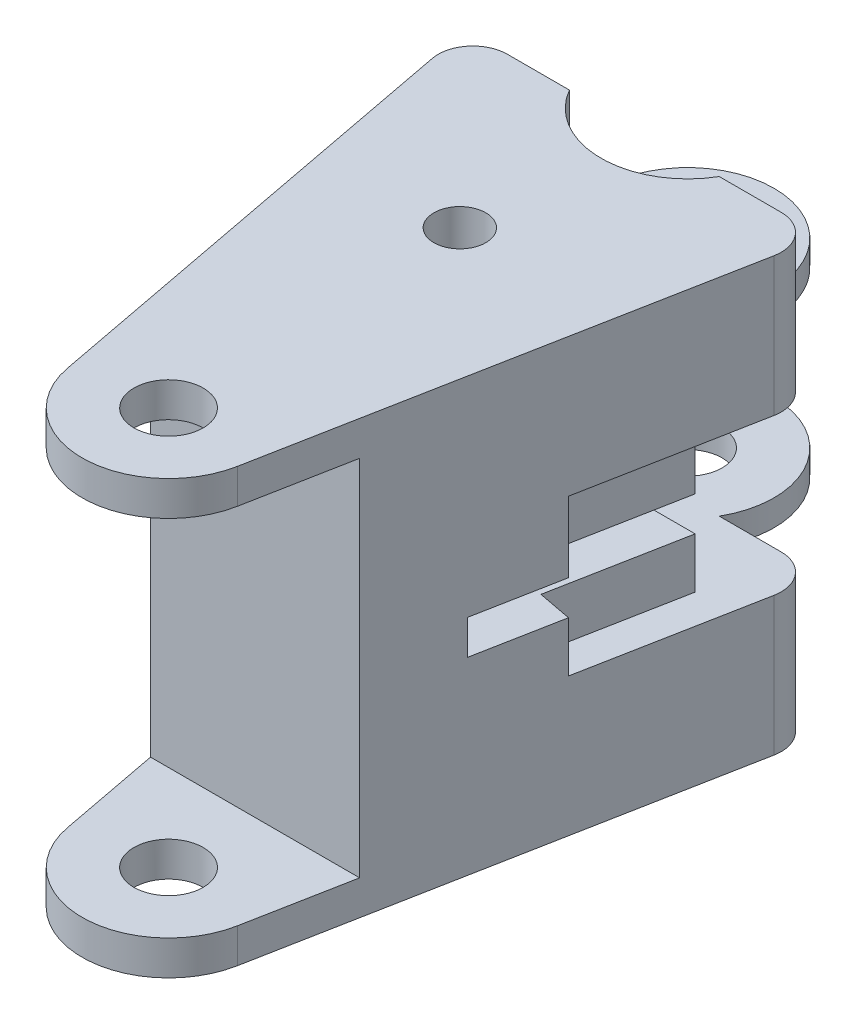
SolidWorks part; units mm, degrees
ref_plane "Front Plane" through (0, 0, 0) normal (0, 0, 1) x (1, 0, 0)
ref_plane "Top Plane" through (0, 0, 0) normal (0, 1, 0) x (1, 0, 0)
ref_plane "Right Plane" through (0, 0, 0) normal (1, 0, 0) x (0, 0, -1)
other "Configuration Table"
sketch "Sketch1" plane through (0, 0, 0) normal (0, 1, 0) x (1, 0, 0)
  line L0 (-4.3301, -2.5) -> (-10.3301, -2.5)
  line L1 (-10.3301, -2.5) -> (-4.9116, -30.9359)
  line L2 (0, 0) -> (0, -50000) construction
  line L3 (10.3301, -2.5) -> (4.9116, -30.9359)
  line L4 (4.3301, -2.5) -> (10.3301, -2.5)
  arc A0 (4.3301, -2.5) -> (-4.3301, -2.5) centre (0, 0) ccw
  arc A1 (-4.9116, -30.9359) -> (4.9116, -30.9359) centre (0, -30) ccw
  dimension "D1" = 10
  dimension "D2" = 10
  dimension "D3" = 30
  dimension "D4" = 6
  dimension "D5" = 2.5
extrude "Boss-Extrude1" add sketch "Sketch1" along normal blind 25
sketch "Sketch2" plane through (0, 25, 0) normal (0, 1, 0) x (1, 0, 0)
  circle A0 centre (0, 0) radius 2
  circle A1 centre (0, -30) radius 2
  dimension "D1" = 4
  dimension "D2" = 4
extrude "Cut-Extrude1" cut sketch "Sketch2" against normal through all
fillet "Fillet1" radius 2 1 edges at (10.3301, 12.5, 2.5)
fillet "Fillet2" radius 2 1 edges at (-10.3301, 12.5, 2.5)
sketch "Sketch3" plane through (0, 25, 0) normal (0, 1, 0) x (1, 0, 0)
  circle A0 centre (0, 0) radius 5
  dimension "D1" = 10
extrude "Cut-Extrude2" cut sketch "Sketch3" against normal blind 6.5
sketch "Sketch4" plane through (0, 0, 0) normal (0, -1, 0) x (1, 0, 0)
  circle A0 centre (0, 0) radius 5
  dimension "D1" = 10
extrude "Cut-Extrude3" cut sketch "Sketch4" against normal blind 6.5
sketch "Sketch5" plane through (0, 0, 0) normal (1, 0, 0) x (0, 0, -1)
  line L0 (-35, 23) -> (-25, 23)
  line L1 (-35, 25) -> (-35, 0) construction
  line L2 (-25, 23) -> (-25, 2)
  line L3 (-25, 2) -> (-35, 2)
  line L4 (-35, 2) -> (-35, 23)
  line L5 (-30.9359, 25) -> (-4.8744, 25) construction
  line L6 (-30.9359, 0) -> (-4.8744, 0) construction
  line L7 (-7, 17) -> (5, 17)
  line L8 (5, 6.5) -> (5, 18.5) construction
  line L9 (5, 17) -> (5, 8)
  line L10 (5, 8) -> (-7, 8)
  line L11 (-7, 8) -> (-7, 17)
  line L12 (-2.5, 25) -> (-4.8744, 25) construction
  line L13 (-4.8744, 0) -> (-2.5, 0) construction
  dimension "D1" = 2
  dimension "D2" = 2
  dimension "D3" = 10
  dimension "D4" = 8
  dimension "D5" = 8
  dimension "D6" = 12
extrude "Cut-Extrude4" cut sketch "Sketch5" against normal through all both and the other way through all
sketch "Sketch7" plane through (10.4279, 0, 1.987) normal (0.9823, 0, 0.1872) x (0.1872, 0, -0.9823)
  line L0 (-5.1032, 17) -> (-13.1032, 17)
  line L2 (-5.1032, 17) -> (-5.1032, 8)
  line L3 (-5.1032, 8) -> (-13.1032, 8)
  line L4 (-13.1032, 8) -> (-13.1032, 17)
  dimension "D1" = 8
extrude "Cut-Extrude5" cut sketch "Sketch7" against normal blind 2
extrude "Cut-Extrude6" cut sketch "Sketch8" against normal through all both and the other way through all
sketch "Sketch8" plane through (59.5987, 25, -138.4861) normal (0, 1, 0) x (0.9893, 0, 0.1458)
  circle A0 centre (-37.5399, -158.2081) radius 1.5
sketch "Sketch9" plane through (8.4632, 0, 1.6127) normal (0.9823, 0, 0.1872) x (0.1872, 0, -0.9823)
  line L0 (-5.4843, 17) -> (-5.4843, 8) construction
  line L1 (-5.4843, 12.9172) -> (-18.1032, 12.9172)
  line L2 (-5.4843, 12.9172) -> (-5.4843, 10.9172)
  line L3 (-5.4843, 10.9172) -> (-18.1032, 10.9172)
  line L4 (-18.1032, 12.9172) -> (-18.1032, 10.9172)
  dimension "D1" = 2
extrude "Cut-Extrude7" cut sketch "Sketch9" against normal through all both and the other way through all
